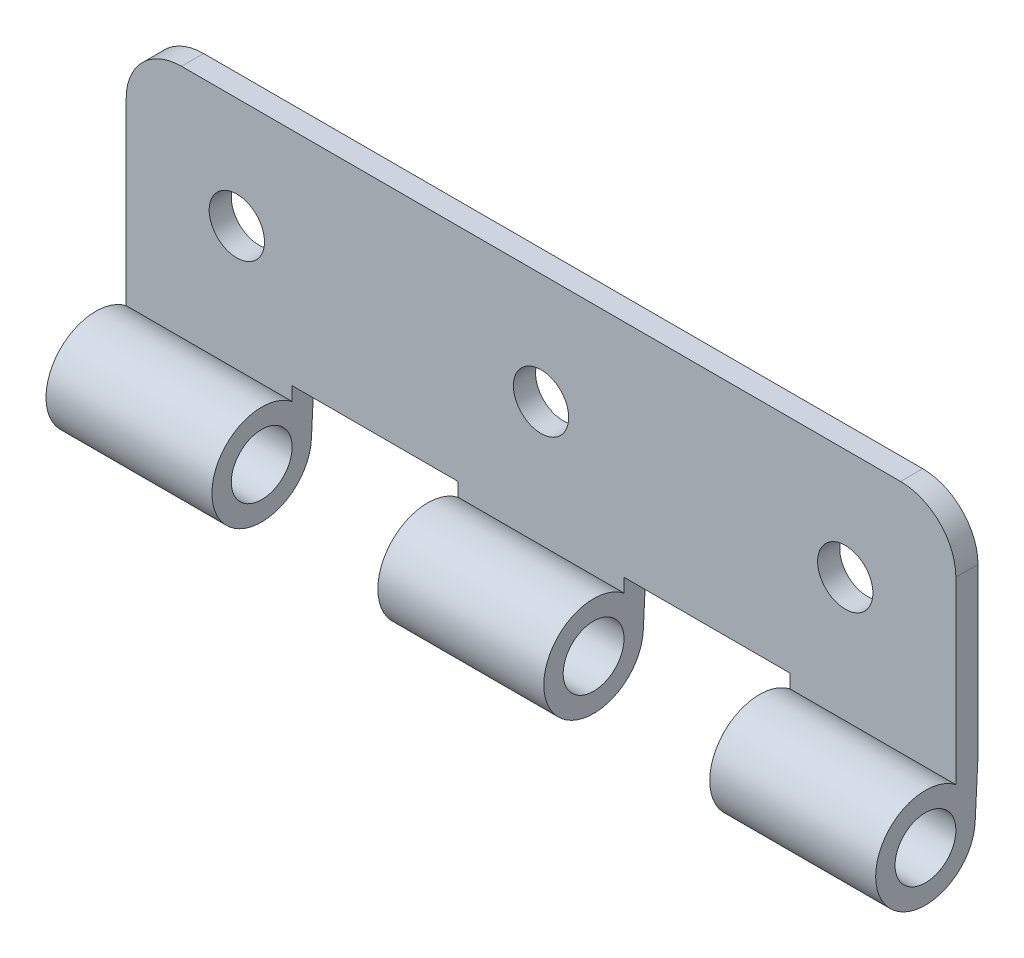
from build123d import *

# Parameters (mm, degrees)
SKETCH1_W           = 75
SKETCH1_H           = 20
SKETCH1_R           = 2.5
BOSS_EXTRUDE1_DEPTH = 2
BOSS_EXTRUDE2_DEPTH = 15
LPATTERN1_COUNT     = 3
LPATTERN1_PITCH     = 30
FILLET1_R           = 5


with BuildPart() as part:
    # Sketch1 → Boss-Extrude1 (new body)
    with BuildSketch(Plane.XY):
        with Locations((37.5, -10)):
            Rectangle(SKETCH1_W, SKETCH1_H)
        with Locations((10, -10)):
            Circle(SKETCH1_R, mode=Mode.SUBTRACT)
        with Locations((65, -10)):
            Circle(SKETCH1_R, mode=Mode.SUBTRACT)
        with Locations((37.5, -10)):
            Circle(SKETCH1_R, mode=Mode.SUBTRACT)
    extrude(amount=BOSS_EXTRUDE1_DEPTH)

    # Sketch2 → Boss-Extrude2 (add)
    # profile 1 of 2: a face of its own
    with BuildSketch(Plane.ZY):
        with BuildLine():
            ThreePointArc((2, -28.361951712), (9.25, -24.8), (2, -21.238048288))
            Line((2, -21.238048288), (2, -24.8))
            Line((2, -24.8), (2, -28.361951712))
        make_face()
        with BuildLine():
            ThreePointArc((7.5, -24.8), (4.75, -27.55), (2, -24.8))
            ThreePointArc((2, -24.8), (4.75, -22.05), (7.5, -24.8))
        make_face(mode=Mode.SUBTRACT)
    # profile 2 of 2: a face of its own
    with BuildSketch(Plane.ZY):
        with BuildLine():
            Line((2, -21.238048288), (2, -20))
            Line((2, -20), (0, -20))
            Line((0, -20), (0.255811418, -25.028624118))
            ThreePointArc((0.255811418, -25.028624118), (0.762853744, -26.886304085), (2, -28.361951712))
            Line((2, -28.361951712), (2, -24.8))
            Line((2, -24.8), (2, -21.238048288))
        make_face()
    boss_extrude2 = extrude(amount=-BOSS_EXTRUDE2_DEPTH)

    # LPattern1: Boss-Extrude2 ×3
    with Locations(*[(i * LPATTERN1_PITCH, 0, 0) for i in range(1, LPATTERN1_COUNT)]):
        add(boss_extrude2)

    # Fillet1
    fillet1_edges = [part.edges().sort_by_distance(p)[0] for p in [
        (0, 0, 1),
        (75, 0, 1),
    ]]
    fillet(fillet1_edges, radius=FILLET1_R)


solid = part.part
